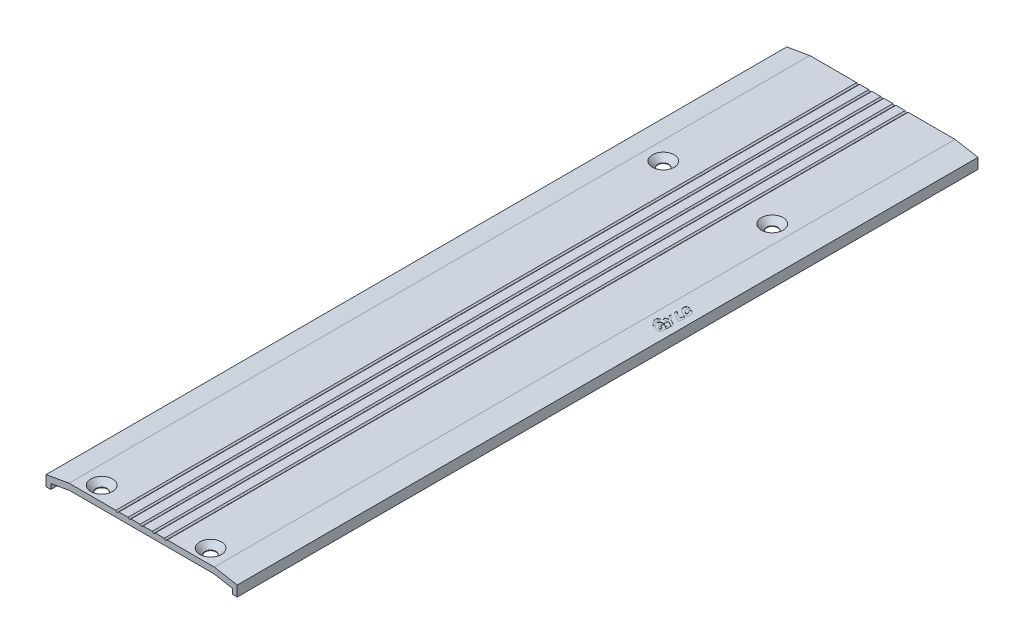
from build123d import *

# Parameters (mm, degrees)
EXTRUDE_1_DEPTH           = 250
CUT_EXTRUDE_1_DEPTH       = 0.1
EXTRUDE_2_DEPTH           = 23
EXTRUDE_3_DEPTH           = 23
HOLE_WIZARD_0_D           = 4.5
HOLE_WIZARD_0_CSINK_D     = 9
HOLE_WIZARD_0_CSINK_ANGLE = 90
EXTRUDE_4_DEPTH           = 10


with BuildPart() as part:
    # Model → 凸台-拉伸1 (new body)
    with BuildSketch(Plane.XY):
        Polygon((2831.092215663, 745.101578786), (2821.592215663, 743.426472469), (2821.592215663, 739.101578786), (2823.592215663, 739.101578786), (2823.592215663, 741.240559901), (2831.310937322, 742.601578786), (2890.873494004, 742.601578786), (2898.592215663, 741.240559901), (2898.592215663, 739.101578786), (2900.592215663, 739.101578786), (2900.592215663, 743.426472469), (2891.092215663, 745.101578786), (2871.710252666, 745.101578786), (2871.092215663, 744.601578786), (2870.474178661, 745.101578786), (2866.710252666, 745.101578786), (2866.092215663, 744.601578786), (2865.474178661, 745.101578786), (2861.710252666, 745.101578786), (2861.092215663, 744.601578786), (2860.474178661, 745.101578786), (2856.710252666, 745.101578786), (2856.092215663, 744.601578786), (2855.474178661, 745.101578786), (2851.710252666, 745.101578786), (2851.092215663, 744.601578786), (2850.474178661, 745.101578786), align=None)
    extrude(amount=EXTRUDE_1_DEPTH)

    # 草图1 → 切除-拉伸1 (cut)
    with BuildSketch(Plane(origin=(214.596971693, 1217.039904055, 0), x_dir=(0.9848077530109746, -0.1736481776739262, 0), z_dir=(0.17364817767392618, 0.9848077530109745, 0))):
        with BuildLine():
            Line((2722.813350585, -82.272677588), (2722.813350585, -81.272677588))
            add(Edge.make_bspline(
                [(2722.813350585, -81.272677588), (2720.098395425, -80.891367095), (2721.539488829, -83.466805597), (2722.980582232, -86.042244099), (2724.536289142, -84.351813392), (2726.091996051, -82.661382685), (2723.399456691, -81.445765021)],
                knots=[2.310776883, 2.310776883, 2.310776883, 4.295504112, 4.295504112, 6.280231341, 6.280231341, 8.26495857, 8.26495857, 8.26495857], degree=2, weights=[1, 0.546712287, 1, 0.546712287, 1, 0.546712287, 1]))
            Line((2723.399456691, -81.445765021), (2723.399456691, -82.630759165))
            add(Edge.make_bspline(
                [(2722.813350585, -82.272677588), (2721.79043745, -81.943078281), (2722.387154928, -82.959375958), (2722.983872407, -83.975673634), (2723.680485897, -83.749536627), (2724.377099386, -83.523399621), (2723.399456691, -82.630759165)],
                knots=[5.452369537, 5.452369537, 5.452369537, 7.300104454, 7.300104454, 9.147839371, 9.147839371, 10.995574288, 10.995574288, 10.995574288], degree=2, weights=[1, 0.602738677, 1, 0.602738677, 1, 0.602738677, 1]))
        make_face()
        Polygon((2723.947967705, -86.704133005), (2721.272244062, -85.441972142), (2721.272244062, -86.441972142), (2724.852395767, -88.130759165), (2724.852395767, -85.630759165), (2723.947967705, -85.204133005), align=None)
        Polygon((2722.973010525, -89.446718879), (2724.852395767, -90.130759165), (2724.852395767, -91.130759165), (2722.973010525, -90.446718879), (2721.272244062, -91.130759165), (2721.272244062, -90.130759165), (2722.29270394, -89.720334993), (2721.272244062, -88.630759165), (2721.272244062, -87.630759165), align=None)
        with BuildLine():
            Line((2722.746954699, -93.253746163), (2722.659798957, -92.257551464))
            add(Edge.make_bspline(
                [(2722.659798957, -92.257551464), (2717.490591073, -91.968672054), (2722.325768389, -95.327168138), (2727.160945704, -98.685664222), (2724.636785845, -93.630759165)],
                knots=[5.539635999, 5.539635999, 5.539635999, 8.030367113, 8.030367113, 10.521098226, 10.521098226, 10.521098226], degree=2, weights=[1, 0.319716976, 1, 0.319716976, 1]))
            Line((2724.636785845, -93.630759165), (2724.852395767, -93.630759165))
            Line((2724.852395767, -93.630759165), (2724.852395767, -93.130759165))
            Line((2724.852395767, -93.130759165), (2723.008853275, -92.261145))
            Line((2723.008853275, -92.261145), (2723.008853275, -93.951182078))
            Line((2723.008853275, -93.951182078), (2723.452769952, -94.181264637))
            Line((2723.452769952, -94.181264637), (2723.452769952, -93.681264637))
            add(Edge.make_bspline(
                [(2722.746954699, -93.253746163), (2721.809951026, -93.022473901), (2722.402716181, -93.98524995), (2722.995481336, -94.948025999), (2723.669889827, -94.752788115), (2724.344298318, -94.557550231), (2723.452769952, -93.681264637)],
                knots=[5.539635999, 5.539635999, 5.539635999, 7.333784926, 7.333784926, 9.127933854, 9.127933854, 10.922082781, 10.922082781, 10.922082781], degree=2, weights=[1, 0.623898956, 1, 0.623898956, 1, 0.623898956, 1]))
        make_face()
        with BuildLine():
            add(Edge.make_bspline(
                [(2720.98702462, -92.608909027), (2719.756792423, -94.341927995), (2722.029380258, -95.712610775)],
                knots=[3.081871514, 3.081871514, 3.081871514, 4.71238898, 4.71238898, 4.71238898], degree=2, weights=[1, 0.685680084, 1]))
            add(Edge.make_bspline(
                [(2720.832240969, -91.620960637), (2717.207188633, -92.804166525), (2722.029380258, -95.712610775)],
                knots=[5.824568949, 5.824568949, 5.824568949, 7.853981634, 7.853981634, 7.853981634], degree=2, weights=[1, 0.527869365, 1]))
            Line((2720.832240969, -91.620960637), (2720.98702462, -92.608909027))
        make_face()
        with BuildLine():
            add(Edge.make_bspline(
                [(2725.137615209, -95.391090973), (2726.367847406, -93.658072005), (2724.095259571, -92.287389225)],
                knots=[3.081871514, 3.081871514, 3.081871514, 4.71238898, 4.71238898, 4.71238898], degree=2, weights=[1, 0.685680084, 1]))
            add(Edge.make_bspline(
                [(2725.29239886, -96.379039363), (2728.917451195, -95.195833475), (2724.095259571, -92.287389225)],
                knots=[2.682976295, 2.682976295, 2.682976295, 4.71238898, 4.71238898, 4.71238898], degree=2, weights=[1, 0.527869365, 1]))
            Line((2725.29239886, -96.379039363), (2725.137615209, -95.391090973))
        make_face()
    extrude(amount=-CUT_EXTRUDE_1_DEPTH, mode=Mode.SUBTRACT)

    # 草图4 → 凸台-拉伸2 (add)
    with BuildSketch(Plane.XY.offset(250)):
        Polygon((2850.474178661, 745.101578786), (2831.092215663, 745.101578786), (2821.592215663, 743.426472469), (2821.592215663, 739.101578786), (2823.592215663, 739.101578786), (2823.592215663, 741.240559901), (2831.310937322, 742.601578786), (2890.873494004, 742.601578786), (2898.592215663, 741.240559901), (2898.592215663, 739.101578786), (2900.592215663, 739.101578786), (2900.592215663, 743.426472469), (2891.092215663, 745.101578786), (2871.710252666, 745.101578786), (2871.092215663, 744.601578786), (2870.474178661, 745.101578786), (2866.710252666, 745.101578786), (2866.092215663, 744.601578786), (2865.474178661, 745.101578786), (2861.710252666, 745.101578786), (2861.092215663, 744.601578786), (2860.474178661, 745.101578786), (2856.710252666, 745.101578786), (2856.092215663, 744.601578786), (2855.474178661, 745.101578786), (2851.710252666, 745.101578786), (2851.092215663, 744.601578786), align=None)
    extrude(amount=EXTRUDE_2_DEPTH)

    # 草图5 → 凸台-拉伸3 (add)
    with BuildSketch(Plane(origin=(0, 0, 0), x_dir=(-1, 0, 0), z_dir=(0, 0, -1))):
        Polygon((-2831.092215663, 745.101578786), (-2850.474178661, 745.101578786), (-2851.092215663, 744.601578786), (-2851.710252666, 745.101578786), (-2855.474178661, 745.101578786), (-2856.092215663, 744.601578786), (-2856.710252666, 745.101578786), (-2860.474178661, 745.101578786), (-2861.092215663, 744.601578786), (-2861.710252666, 745.101578786), (-2865.474178661, 745.101578786), (-2866.092215663, 744.601578786), (-2866.710252666, 745.101578786), (-2870.474178661, 745.101578786), (-2871.092215663, 744.601578786), (-2871.710252666, 745.101578786), (-2891.092215663, 745.101578786), (-2900.592215663, 743.426472469), (-2900.592215663, 739.101578786), (-2898.592215663, 739.101578786), (-2898.592215663, 741.240559901), (-2890.873494004, 742.601578786), (-2831.310937322, 742.601578786), (-2823.592215663, 741.240559901), (-2823.592215663, 739.101578786), (-2821.592215663, 739.101578786), (-2821.592215663, 743.426472469), align=None)
    extrude(amount=EXTRUDE_3_DEPTH)

    # 打孔尺寸(%根据)开槽半沉头木螺钉的类型0 (through all)
    with Locations(Plane(origin=(0, 745.101578786, 0), x_dir=(1, 0, 0), z_dir=(0, 1, 0))):
        with Locations((2883.592215663, -267), (2838.592215663, -267), (2838.592215663, -35), (2883.592215663, -35)):
            CounterSinkHole(HOLE_WIZARD_0_D / 2, HOLE_WIZARD_0_CSINK_D / 2, counter_sink_angle=HOLE_WIZARD_0_CSINK_ANGLE)

    # 草图10 → 凸台-拉伸4 (add)
    with BuildSketch(Plane(origin=(0, 0, -23), x_dir=(-1, 0, 0), z_dir=(0, 0, -1))):
        Polygon((-2821.592215663, 743.426472469), (-2831.092215663, 745.101578786), (-2850.474178661, 745.101578786), (-2851.092215663, 744.601578786), (-2851.710252666, 745.101578786), (-2855.474178661, 745.101578786), (-2856.092215663, 744.601578786), (-2856.710252666, 745.101578786), (-2860.474178661, 745.101578786), (-2861.092215663, 744.601578786), (-2861.710252666, 745.101578786), (-2865.474178661, 745.101578786), (-2866.092215663, 744.601578786), (-2866.710252666, 745.101578786), (-2870.474178661, 745.101578786), (-2871.092215663, 744.601578786), (-2871.710252666, 745.101578786), (-2891.092215663, 745.101578786), (-2900.592215663, 743.426472469), (-2900.592215663, 739.101578786), (-2898.592215663, 739.101578786), (-2898.592215663, 741.240559901), (-2890.873494004, 742.601578786), (-2831.310937322, 742.601578786), (-2823.592215663, 741.240559901), (-2823.592215663, 739.101578786), (-2821.592215663, 739.101578786), align=None)
    extrude(amount=EXTRUDE_4_DEPTH)


solid = part.part
